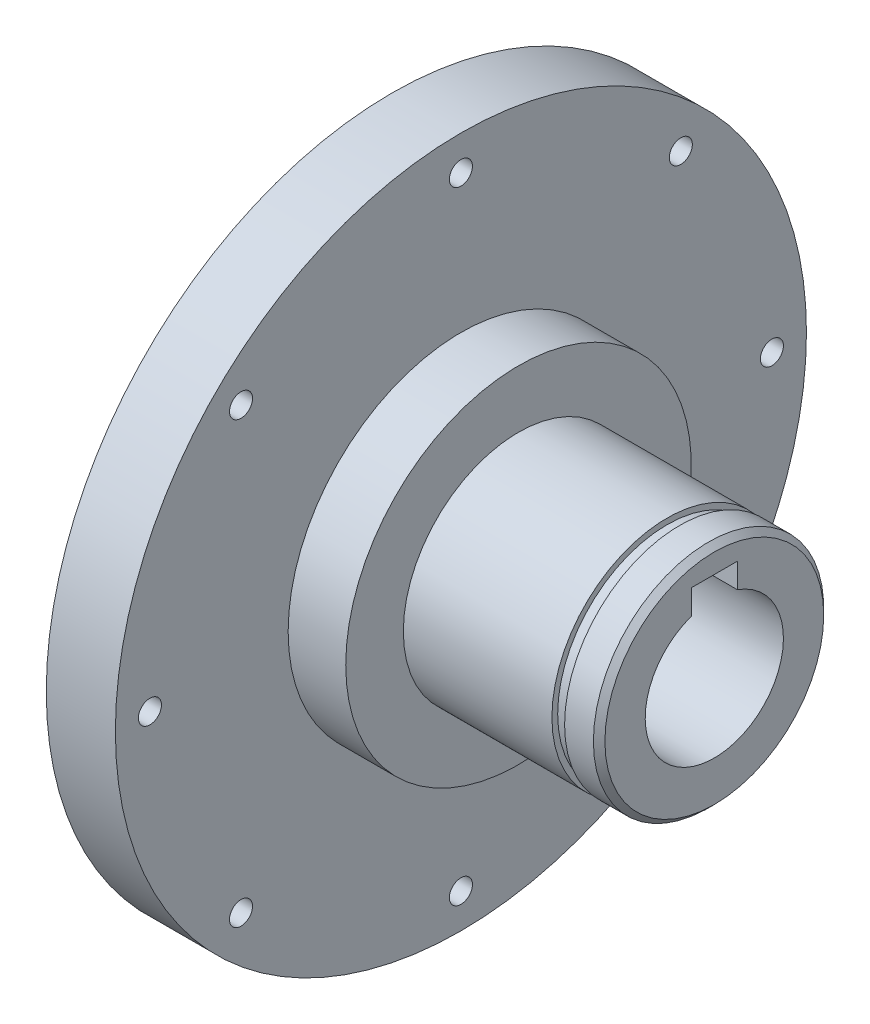
from build123d import *

# Parameters (mm, degrees)
SKETCH_1_W          = 12
SKETCH_1_H          = 60
SKETCH_2_W          = 10
SKETCH_2_H          = 30
SKETCH_3_W          = 34
SKETCH_3_H          = 20
CUT_EXTRUDE_2_DEPTH = 102.666120217
CUT_EXTRUDE_START   = 50
SKETCH_6_OUTSIDE_W  = 157.742
SKETCH_6_OUTSIDE_H  = 157.742
SKETCH_6_OUTSIDE_R  = 19
CUT_EXTRUDE_4_DEPTH = 2.2
SKETCH_7_R          = 2
CUT_EXTRUDE_5_DEPTH = 102.666120217
CHAMFER_2_SIZE      = 1


with BuildPart() as part:
    # 草图1 → 旋转-薄壁2 (revolve)
    with BuildSketch(Plane.XY, mode=Mode.PRIVATE) as revolve_2_sk:
        with Locations((6, 30)):
            Rectangle(SKETCH_1_W, SKETCH_1_H)
    revolve(revolve_2_sk.sketch.rotate(Axis((0, 0, 0), (1, 0, 0)), 90), axis=Axis((0, 0, 0), (1, 0, 0)))

    # 草图2 → 旋转-薄壁4 (revolve)
    with BuildSketch(Plane.XY, mode=Mode.PRIVATE) as revolve_4_sk:
        with Locations((17, 15)):
            Rectangle(SKETCH_2_W, SKETCH_2_H)
    revolve(revolve_4_sk.sketch.rotate(Axis((12, 0, 0), (1, 0, 0)), 90), axis=Axis((12, 0, 0), (1, 0, 0)))

    # 草图3 → 旋转-薄壁5 (revolve)
    with BuildSketch(Plane.XY, mode=Mode.PRIVATE) as revolve_5_sk:
        with Locations((39, 10)):
            Rectangle(SKETCH_3_W, SKETCH_3_H)
    revolve(revolve_5_sk.sketch.rotate(Axis((22, 0, 0), (1, 0, 0)), 90), axis=Axis((22, 0, 0), (1, 0, 0)))

    # 草图4 → 切除-拉伸2 (cut, through all)
    with BuildSketch(Plane(origin=(0, 0, 0), x_dir=(0, 0, -1), z_dir=(1, 0, 0))):
        with BuildLine():
            Line((-4, 15.6), (4, 15.6))
            Line((4, 15.6), (4, 11.313708499))
            ThreePointArc((4, 11.313708499), (0, -12), (-4, 11.313708499))
            Line((-4, 11.313708499), (-4, 15.6))
        make_face()
    extrude(amount=CUT_EXTRUDE_2_DEPTH, mode=Mode.SUBTRACT)

    # 草图6 outside → 切除-拉伸4 (cut)
    with BuildSketch(Plane(origin=(0, 0, 0), x_dir=(0, 0, -1), z_dir=(1, 0, 0)).offset(CUT_EXTRUDE_START)):
        Rectangle(SKETCH_6_OUTSIDE_W, SKETCH_6_OUTSIDE_H)
        Circle(SKETCH_6_OUTSIDE_R, mode=Mode.SUBTRACT)
    extrude(amount=-CUT_EXTRUDE_4_DEPTH, mode=Mode.SUBTRACT)

    # 草图7 → 切除-拉伸5 (cut, through all)
    with BuildSketch(Plane.ZY):
        with Locations((0, 54)):
            Circle(SKETCH_7_R)
        with Locations((38.183766184, 38.183766184)):
            Circle(SKETCH_7_R)
        with Locations((54, 0)):
            Circle(SKETCH_7_R)
        with Locations((38.183766184, -38.183766184)):
            Circle(SKETCH_7_R)
        with Locations((0, -54)):
            Circle(SKETCH_7_R)
        with Locations((-38.183766184, -38.183766184)):
            Circle(SKETCH_7_R)
        with Locations((-54, 0)):
            Circle(SKETCH_7_R)
        with Locations((-38.183766184, 38.183766184)):
            Circle(SKETCH_7_R)
    extrude(amount=-CUT_EXTRUDE_5_DEPTH, mode=Mode.SUBTRACT)

    # 倒角2
    chamfer_2_edges = [part.edges().sort_by_distance(p)[0] for p in [
        (56, 0, -20),
    ]]
    chamfer(chamfer_2_edges, length=CHAMFER_2_SIZE)


solid = part.part
